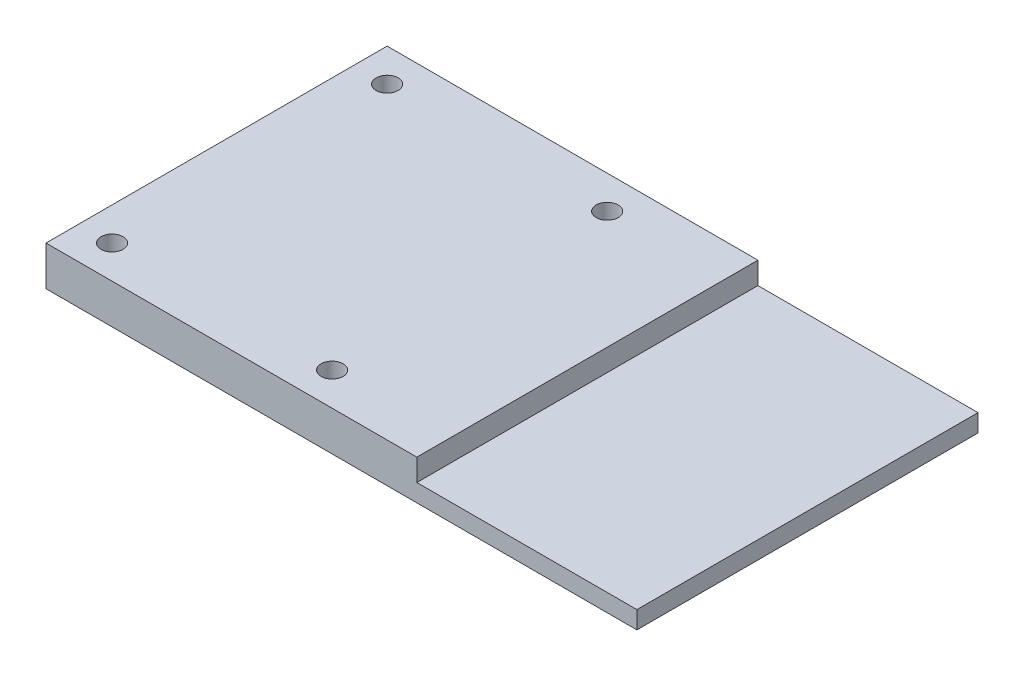
SolidWorks part; units mm, degrees
material "普通碳钢"
ref_plane "Front Plane" through (0, 0, 0) normal (0, 0, 1) x (1, 0, 0)
ref_plane "Top Plane" through (0, 0, 0) normal (0, 1, 0) x (1, 0, 0)
ref_plane "Right Plane" through (0, 0, 0) normal (1, 0, 0) x (0, 0, -1)
sketch "Sketch1" plane through (0, 0, 0) normal (0, 1, 0) x (1, 0, 0)
  line L1 (-134.25, -77.5) -> (134.25, -77.5)
  line L2 (-134.25, -77.5) -> (-134.25, 77.5)
  line L3 (-134.25, 77.5) -> (134.25, 77.5)
  line L4 (134.25, -77.5) -> (134.25, 77.5)
  line L5 (-134.25, -77.5) -> (134.25, 77.5) construction
  line L6 (-134.25, 77.5) -> (134.25, -77.5) construction
  point P0 (0, 0)
  dimension "D1" = 268.5
  dimension "D2" = 155
extrude "Boss-Extrude1" add sketch "Sketch1" along normal blind 18
sketch "Sketch2" plane through (0, 18, 0) normal (0, 1, 0) x (1, 0, 0)
  line L0 (-134.25, 0) -> (134.25, 0) construction
  line L1 (-134.25, 77.5) -> (-134.25, -77.5) construction
  line L2 (134.25, -77.5) -> (134.25, 77.5) construction
  line L3 (134.25, 77.5) -> (-134.25, 77.5) construction
  circle A0 centre (-119.25, 62.5) radius 5
  circle A1 centre (-19.25, 62.5) radius 5
  circle A2 centre (-19.25, -62.5) radius 5
  circle A3 centre (-119.25, -62.5) radius 5
  dimension "D1" = 15
  dimension "D3" = 100
  dimension "D2" = 15
extrude "Cut-Extrude1" cut sketch "Sketch2" against normal blind 18
sketch "Sketch3" plane through (0, 18, 0) normal (0, 1, 0) x (1, 0, 0)
  line L0 (-134.25, -77.5) -> (134.25, -77.5) construction
  line L1 (134.25, 77.5) -> (34.25, 77.5)
  line L2 (134.25, 77.5) -> (134.25, -77.5)
  line L3 (134.25, -77.5) -> (34.25, -77.5)
  line L4 (34.25, 77.5) -> (34.25, -77.5)
  dimension "D1" = 100
extrude "Cut-Extrude2" cut sketch "Sketch3" against normal blind 10
